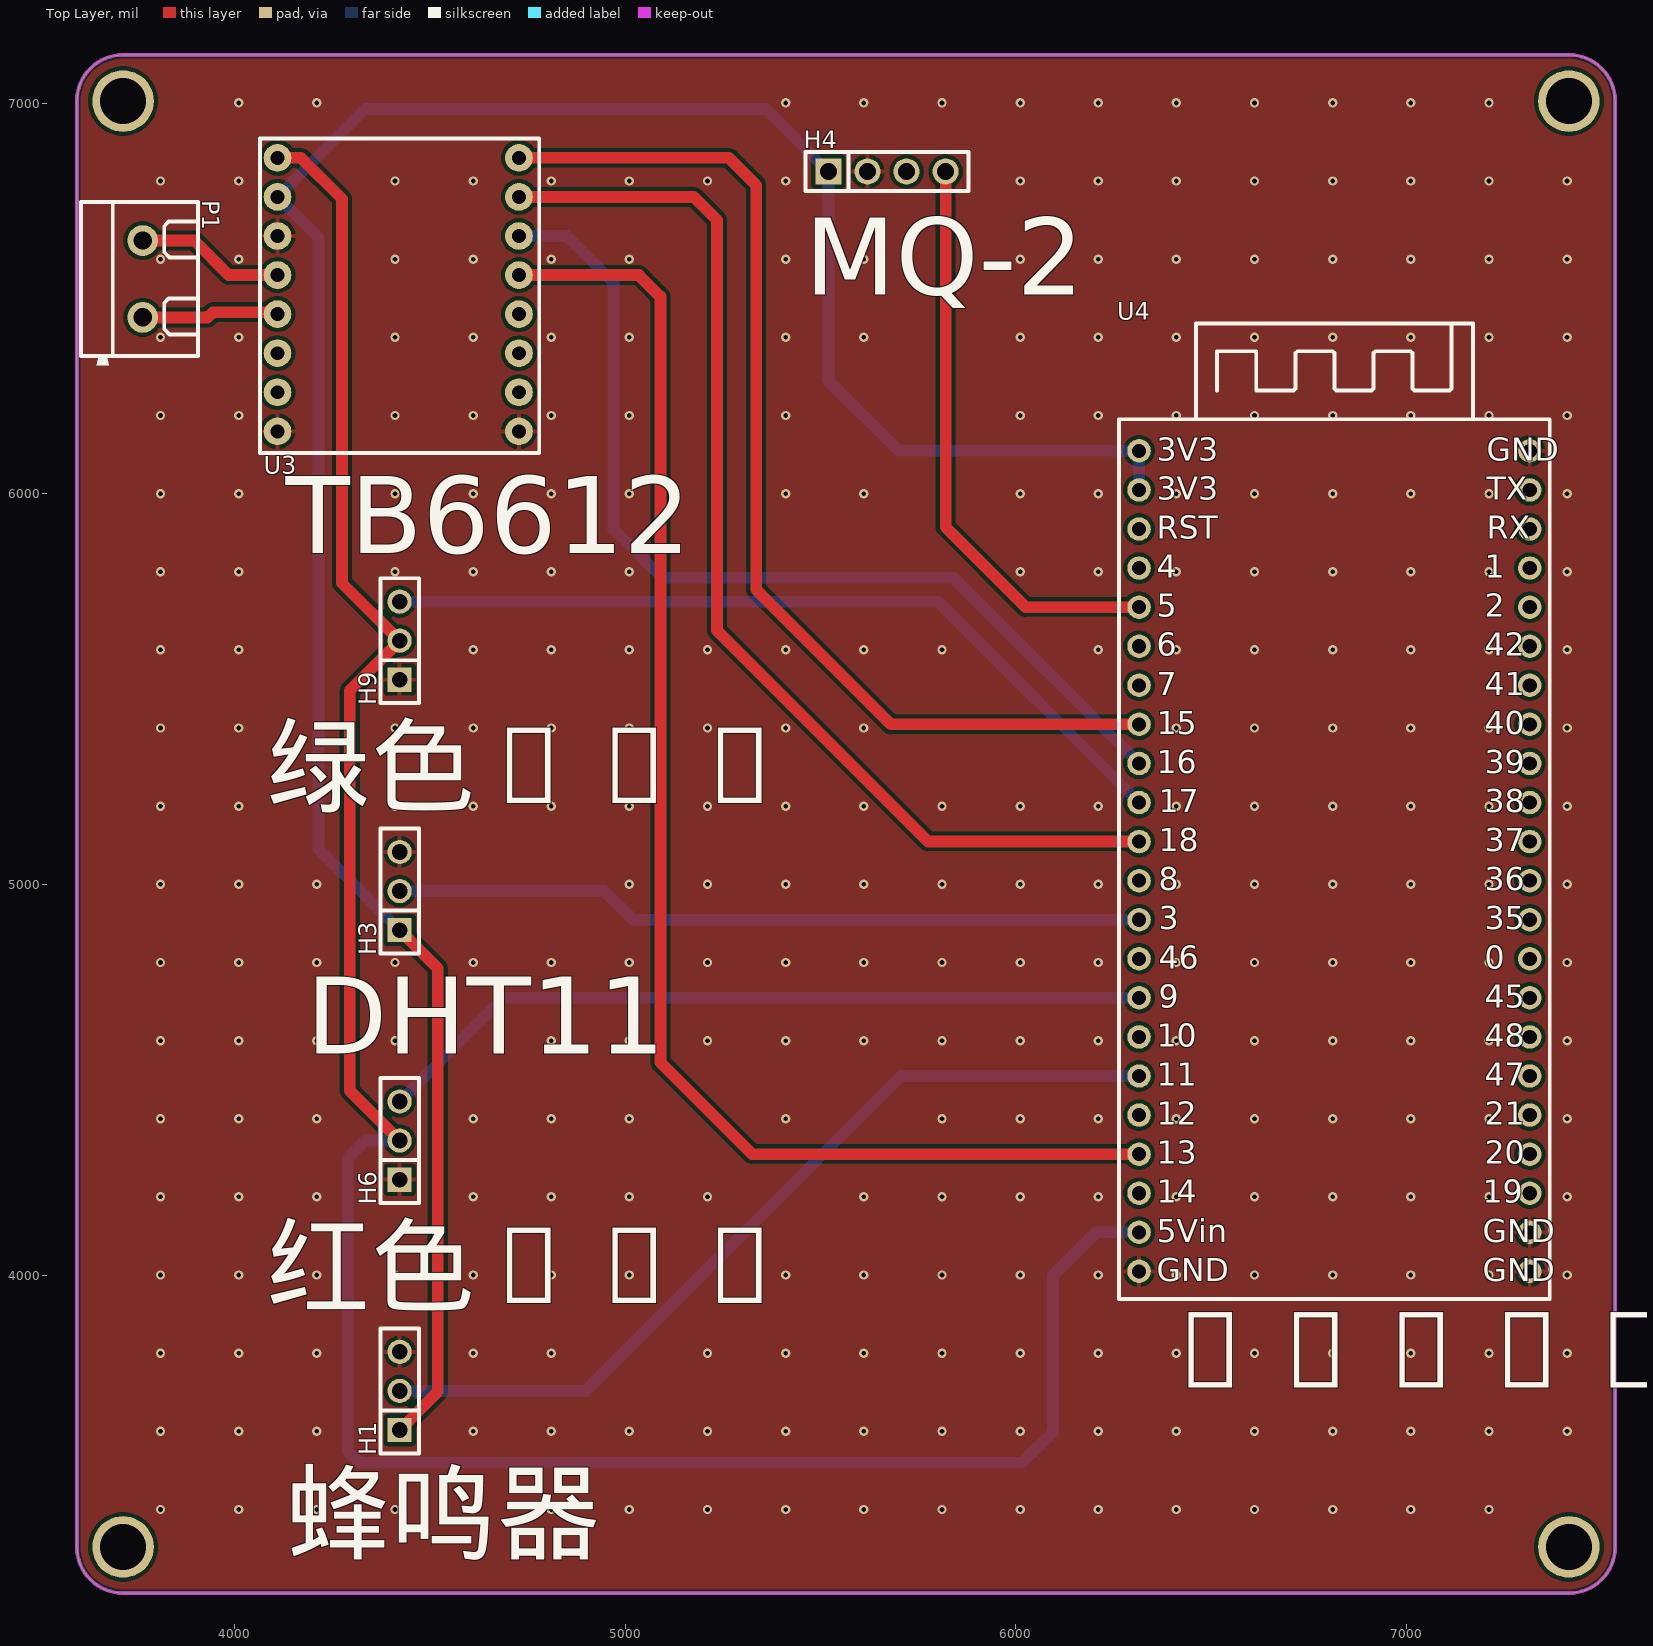
[diagram p0: Top Layer view]
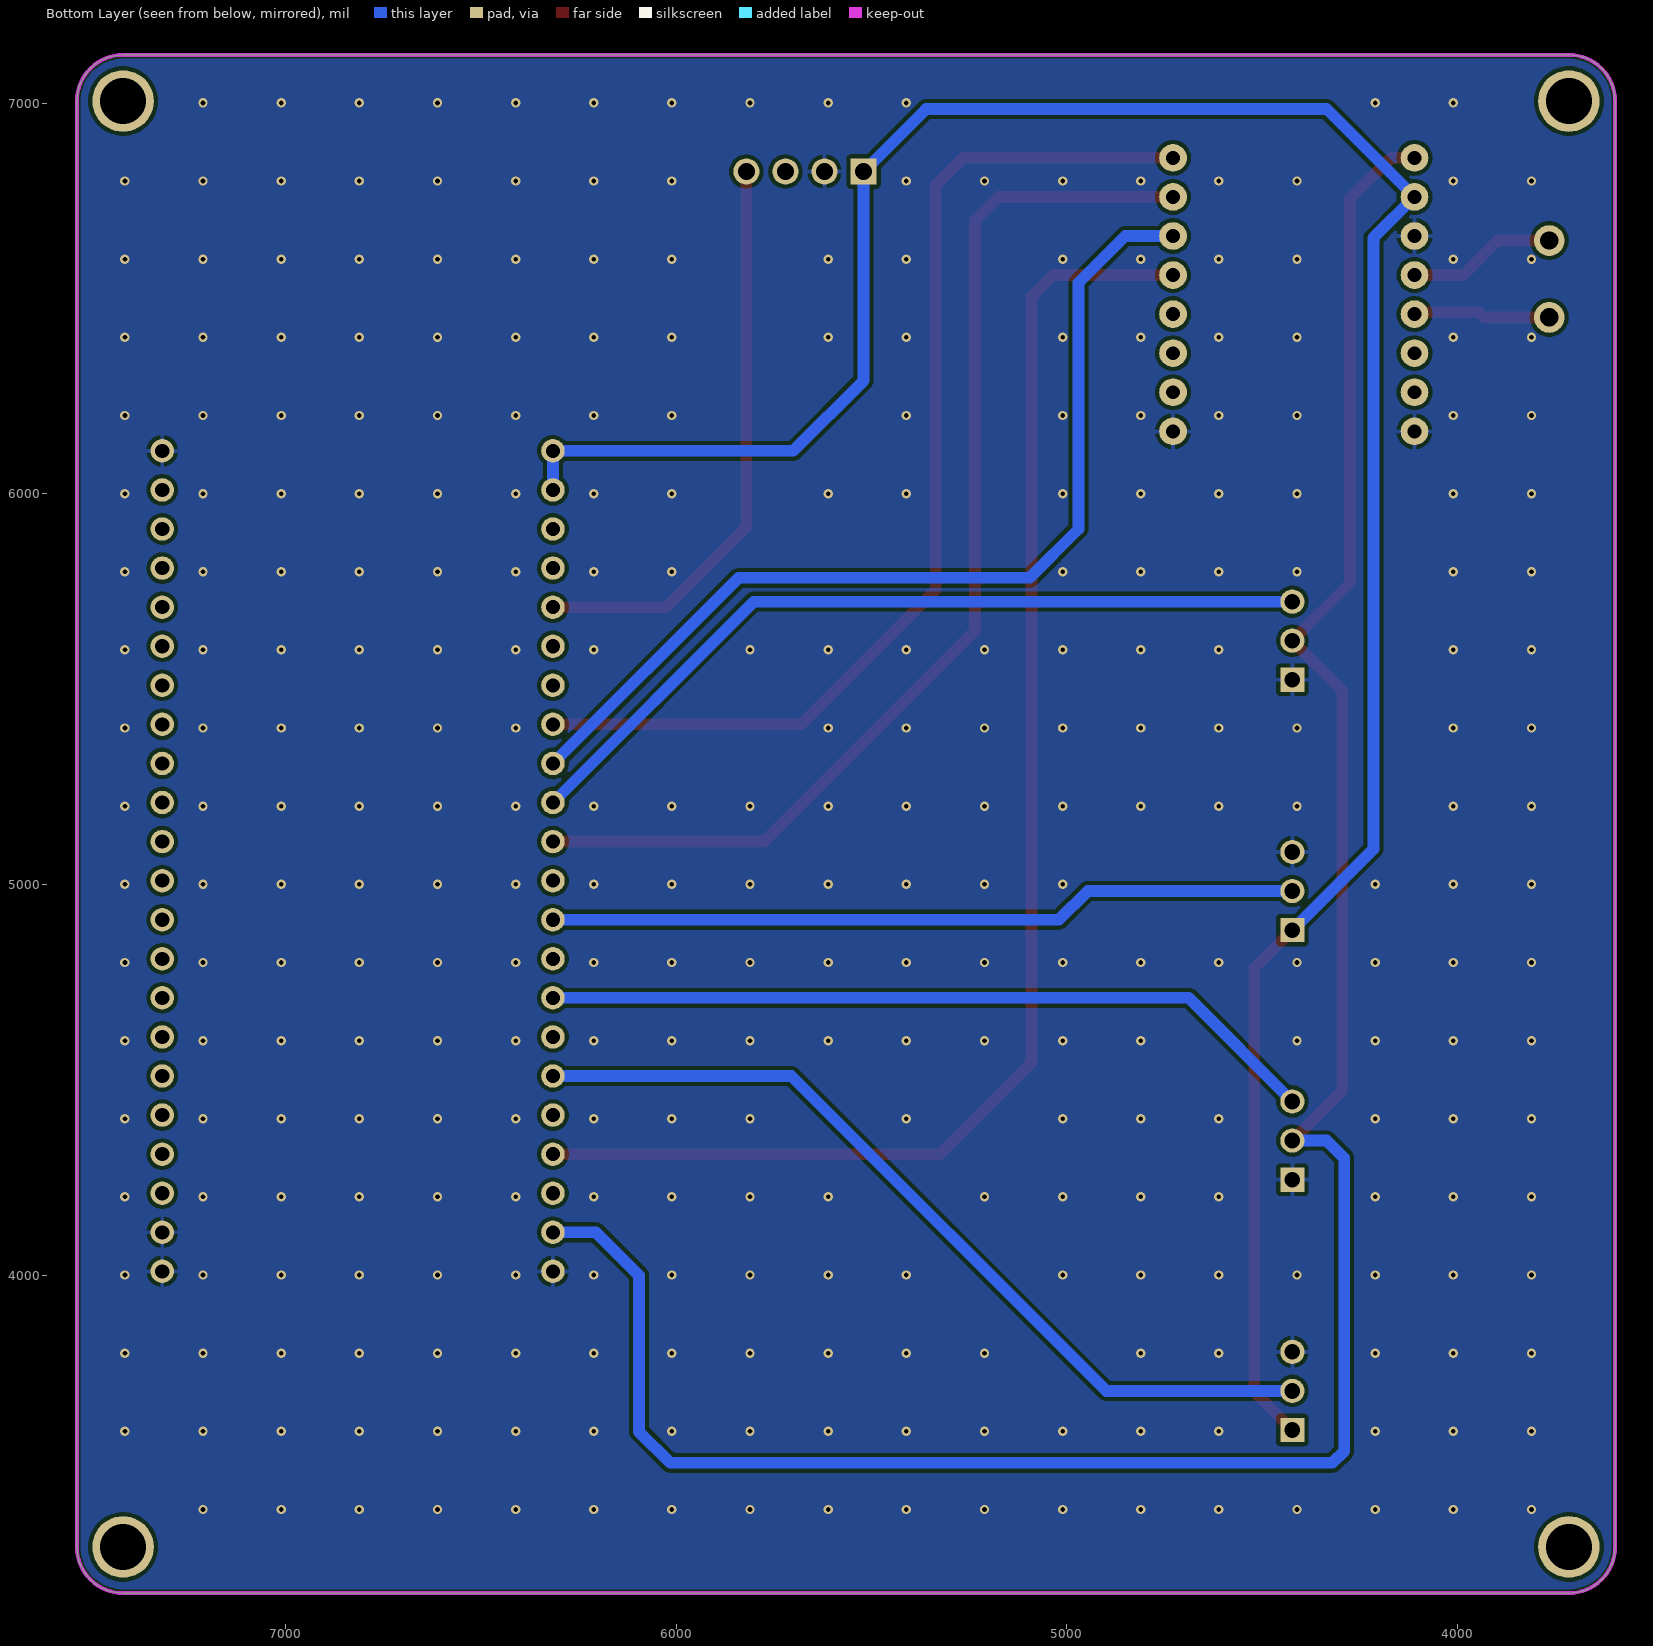
[diagram p1: Bottom Layer view, seen from below]
# Altium PCB MISC52005.pcbdoc
Units mil, origin at the board's own origin, x right, y up, seen from the top; angles counter-clockwise.
Board outline 3937.01 x 3937.01 mil, 2 copper layers (Top Layer, Bottom Layer), stack 62.206 mil thick; 8 components, 42 nets, 82 pads, 311 vias.

## Layer stack, top to bottom
Top Solder Mask Layer: solder mask 0.394, Dk 3.3
Top Layer: signal copper 1.379
Dielectric1: surface 59.449, FR4, Dk 4.5
Bottom Layer: signal copper 1.378
Bottom Solder Mask Layer: solder mask 0.394, Dk 3.3

## Board outline
3714.61,7123.5 ccw(c3714.61,7005.39) 3596.5,7005.39 3596.5,3304.61 ccw(c3714.61,3304.61) 3714.61,3186.5 7415.39,3186.5 ccw(c7415.39,3304.61) 7533.5,3304.61 7533.5,7005.39 ccw(c7415.39,7005.39) 7415.39,7123.5 3714.61,7123.5

## Design rules (kind name [scope] priority, off if disabled: settings)
BoardOutlineClearance copperThickness2oz_1 [All] p2 off: genericclearance=7.99 ignorepadtopadclearanceinfootprint=FALSE except(0: Arc-SplitContinuation Track-SplitContinuation SMDPad-SplitContinuation THPad-SplitContinuation Via-SplitContinuation Fill-SplitContinuation Region-SplitContinuation Poly-SplitContinuation Text-SplitContinuation Hole-SplitContinuation; 5.98: Arc-CutoutEdge Track-CutoutEdge SMDPad-CutoutEdge THPad-CutoutEdge Via-CutoutEdge Text-CutoutEdge; 6.9: Hole-OutlineEdge Hole-CutoutEdge; 10: Poly-OutlineEdge Poly-CutoutEdge; 11.81: Arc-OutlineEdge Track-OutlineEdge SMDPad-OutlineEdge THPad-OutlineEdge Via-OutlineEdge Fill-OutlineEdge Region-OutlineEdge Text-OutlineEdge Fill-CutoutEdge Region-CutoutEdge)
BoardOutlineClearance Plane_innerPlane_1 [All] p4 off: genericclearance=4.02 ignorepadtopadclearanceinfootprint=FALSE except(0: Arc-SplitContinuation Track-SplitContinuation SMDPad-SplitContinuation THPad-SplitContinuation Via-SplitContinuation Fill-SplitContinuation Region-SplitContinuation Poly-SplitContinuation Text-SplitContinuation Hole-SplitContinuation; 5.98: Arc-CutoutEdge Track-CutoutEdge SMDPad-CutoutEdge THPad-CutoutEdge Via-CutoutEdge Text-CutoutEdge; 6.9: Hole-OutlineEdge Hole-CutoutEdge; 10: Poly-OutlineEdge Poly-CutoutEdge; 11.81: Arc-OutlineEdge Track-OutlineEdge SMDPad-OutlineEdge THPad-OutlineEdge Via-OutlineEdge Fill-OutlineEdge Region-OutlineEdge Text-OutlineEdge Fill-CutoutEdge Region-CutoutEdge)
BoardOutlineClearance Copper_copperRegion_1 [All] p6 off: genericclearance=4.02 ignorepadtopadclearanceinfootprint=FALSE except(0: Arc-SplitContinuation Track-SplitContinuation SMDPad-SplitContinuation THPad-SplitContinuation Via-SplitContinuation Fill-SplitContinuation Region-SplitContinuation Poly-SplitContinuation Text-SplitContinuation Hole-SplitContinuation; 5.98: Arc-CutoutEdge Track-CutoutEdge SMDPad-CutoutEdge THPad-CutoutEdge Via-CutoutEdge Text-CutoutEdge; 6.9: Hole-OutlineEdge Hole-CutoutEdge; 10: Poly-OutlineEdge Poly-CutoutEdge; 11.81: Arc-OutlineEdge Track-OutlineEdge SMDPad-OutlineEdge THPad-OutlineEdge Via-OutlineEdge Fill-OutlineEdge Region-OutlineEdge Text-OutlineEdge Fill-CutoutEdge Region-CutoutEdge)
BoardOutlineClearance Copper_copperRegion_copperThickness1oz_1 [All] p8 off: genericclearance=4.02 ignorepadtopadclearanceinfootprint=FALSE except(0: Arc-SplitContinuation Track-SplitContinuation SMDPad-SplitContinuation THPad-SplitContinuation Via-SplitContinuation Fill-SplitContinuation Region-SplitContinuation Poly-SplitContinuation Text-SplitContinuation Hole-SplitContinuation; 5.98: Arc-CutoutEdge Track-CutoutEdge SMDPad-CutoutEdge THPad-CutoutEdge Via-CutoutEdge Text-CutoutEdge; 6.9: Hole-OutlineEdge Hole-CutoutEdge; 10: Poly-OutlineEdge Poly-CutoutEdge; 11.81: Arc-OutlineEdge Track-OutlineEdge SMDPad-OutlineEdge THPad-OutlineEdge Via-OutlineEdge Fill-OutlineEdge Region-OutlineEdge Text-OutlineEdge Fill-CutoutEdge Region-CutoutEdge)
BoardOutlineClearance Copper_copperRegion_Copper_copperRegion_1 [All] p10 off: genericclearance=4.02 ignorepadtopadclearanceinfootprint=FALSE except(0: Arc-SplitContinuation Track-SplitContinuation SMDPad-SplitContinuation THPad-SplitContinuation Via-SplitContinuation Fill-SplitContinuation Region-SplitContinuation Poly-SplitContinuation Text-SplitContinuation Hole-SplitContinuation; 5.98: Arc-CutoutEdge Track-CutoutEdge SMDPad-CutoutEdge THPad-CutoutEdge Via-CutoutEdge Text-CutoutEdge; 6.9: Hole-OutlineEdge Hole-CutoutEdge; 10: Poly-OutlineEdge Poly-CutoutEdge; 11.81: Arc-OutlineEdge Track-OutlineEdge SMDPad-OutlineEdge THPad-OutlineEdge Via-OutlineEdge Fill-OutlineEdge Region-OutlineEdge Text-OutlineEdge Fill-CutoutEdge Region-CutoutEdge)
BoardOutlineClearance copperThickness1oz_1 [All] p12: genericclearance=4.02 ignorepadtopadclearanceinfootprint=FALSE except(0: Arc-SplitContinuation Track-SplitContinuation SMDPad-SplitContinuation THPad-SplitContinuation Via-SplitContinuation Fill-SplitContinuation Region-SplitContinuation Poly-SplitContinuation Text-SplitContinuation Hole-SplitContinuation; 5.98: Arc-CutoutEdge Track-CutoutEdge SMDPad-CutoutEdge THPad-CutoutEdge Via-CutoutEdge Text-CutoutEdge; 6.9: Hole-OutlineEdge Hole-CutoutEdge; 10: Poly-OutlineEdge Poly-CutoutEdge; 11.81: Arc-OutlineEdge Track-OutlineEdge SMDPad-OutlineEdge THPad-OutlineEdge Via-OutlineEdge Fill-OutlineEdge Region-OutlineEdge Text-OutlineEdge Fill-CutoutEdge Region-CutoutEdge)
Clearance copperThickness2oz [All] p1 off: gap=7.99 ignorepadtopadclearanceinfootprint=FALSE except(5.98: SMDPad-Track SMDPad-SMDPad THPad-Track SMDPad-THPad THPad-THPad Track-Via SMDPad-Via THPad-Via Via-Via Fill-SMDPad Region-SMDPad Fill-THPad Region-THPad Fill-Via Region-Via Fill-Fill Fill-Region Region-Region Arc-Track Arc-SMDPad Arc-THPad Arc-Via Fill-Arc Region-Arc Arc-Arc Text-Track SMDPad-Text Text-THPad Text-Via Fill-Text Region-Text Arc-Text Text-Text; 6.9: Hole-Track Hole-SMDPad Hole-THPad Hole-Via Fill-Hole Region-Hole Hole-Arc Hole-Text; 10: Poly-Track Poly-SMDPad Poly-THPad Poly-Via Poly-Fill Poly-Region Poly-Poly Poly-Arc Poly-Text Poly-Hole; 11.81: Fill-Track Region-Track)
Clearance Plane_innerPlane [All] p3 off: gap=4.02 ignorepadtopadclearanceinfootprint=FALSE except(5.98: SMDPad-Track SMDPad-SMDPad THPad-Track SMDPad-THPad THPad-THPad Track-Via SMDPad-Via THPad-Via Via-Via Fill-SMDPad Region-SMDPad Fill-THPad Region-THPad Fill-Via Region-Via Fill-Fill Fill-Region Region-Region Arc-Track Arc-SMDPad Arc-THPad Arc-Via Fill-Arc Region-Arc Arc-Arc Text-Track SMDPad-Text Text-THPad Text-Via Fill-Text Region-Text Arc-Text Text-Text; 6.9: Hole-Track Hole-SMDPad Hole-THPad Hole-Via Fill-Hole Region-Hole Hole-Arc Hole-Text; 10: Poly-Track Poly-SMDPad Poly-THPad Poly-Via Poly-Fill Poly-Region Poly-Poly Poly-Arc Poly-Text Poly-Hole; 11.81: Fill-Track Region-Track)
Clearance Copper_copperRegion [All] p5 off: gap=4.02 ignorepadtopadclearanceinfootprint=FALSE except(5.98: SMDPad-Track SMDPad-SMDPad THPad-Track SMDPad-THPad THPad-THPad Track-Via SMDPad-Via THPad-Via Via-Via Fill-SMDPad Region-SMDPad Fill-THPad Region-THPad Fill-Via Region-Via Fill-Fill Fill-Region Region-Region Arc-Track Arc-SMDPad Arc-THPad Arc-Via Fill-Arc Region-Arc Arc-Arc Text-Track SMDPad-Text Text-THPad Text-Via Fill-Text Region-Text Arc-Text Text-Text; 6.9: Hole-Track Hole-SMDPad Hole-THPad Hole-Via Fill-Hole Region-Hole Hole-Arc Hole-Text; 10: Poly-Track Poly-SMDPad Poly-THPad Poly-Via Poly-Fill Poly-Region Poly-Poly Poly-Arc Poly-Text Poly-Hole; 11.81: Fill-Track Region-Track)
Clearance Copper_copperRegion_copperThickness1oz [All] p7 off: gap=4.02 ignorepadtopadclearanceinfootprint=FALSE except(5.98: SMDPad-Track SMDPad-SMDPad THPad-Track SMDPad-THPad THPad-THPad Track-Via SMDPad-Via THPad-Via Via-Via Fill-SMDPad Region-SMDPad Fill-THPad Region-THPad Fill-Via Region-Via Fill-Fill Fill-Region Region-Region Arc-Track Arc-SMDPad Arc-THPad Arc-Via Fill-Arc Region-Arc Arc-Arc Text-Track SMDPad-Text Text-THPad Text-Via Fill-Text Region-Text Arc-Text Text-Text; 6.9: Hole-Track Hole-SMDPad Hole-THPad Hole-Via Fill-Hole Region-Hole Hole-Arc Hole-Text; 10: Poly-Track Poly-SMDPad Poly-THPad Poly-Via Poly-Fill Poly-Region Poly-Poly Poly-Arc Poly-Text Poly-Hole; 11.81: Fill-Track Region-Track)
Clearance Copper_copperRegion_Copper_copperRegion [All] p9 off: gap=4.02 ignorepadtopadclearanceinfootprint=FALSE except(5.98: SMDPad-Track SMDPad-SMDPad THPad-Track SMDPad-THPad THPad-THPad Track-Via SMDPad-Via THPad-Via Via-Via Fill-SMDPad Region-SMDPad Fill-THPad Region-THPad Fill-Via Region-Via Fill-Fill Fill-Region Region-Region Arc-Track Arc-SMDPad Arc-THPad Arc-Via Fill-Arc Region-Arc Arc-Arc Text-Track SMDPad-Text Text-THPad Text-Via Fill-Text Region-Text Arc-Text Text-Text; 6.9: Hole-Track Hole-SMDPad Hole-THPad Hole-Via Fill-Hole Region-Hole Hole-Arc Hole-Text; 10: Poly-Track Poly-SMDPad Poly-THPad Poly-Via Poly-Fill Poly-Region Poly-Poly Poly-Arc Poly-Text Poly-Hole; 11.81: Fill-Track Region-Track)
Clearance copperThickness1oz [All] p11: gap=4.02 ignorepadtopadclearanceinfootprint=FALSE except(5.98: SMDPad-Track SMDPad-SMDPad THPad-Track SMDPad-THPad THPad-THPad Track-Via SMDPad-Via THPad-Via Via-Via Fill-SMDPad Region-SMDPad Fill-THPad Region-THPad Fill-Via Region-Via Fill-Fill Fill-Region Region-Region Arc-Track Arc-SMDPad Arc-THPad Arc-Via Fill-Arc Region-Arc Arc-Arc Text-Track SMDPad-Text Text-THPad Text-Via Fill-Text Region-Text Arc-Text Text-Text; 6.9: Hole-Track Hole-SMDPad Hole-THPad Hole-Via Fill-Hole Region-Hole Hole-Arc Hole-Text; 10: Poly-Track Poly-SMDPad Poly-THPad Poly-Via Poly-Fill Poly-Region Poly-Poly Poly-Arc Poly-Text Poly-Hole; 11.81: Fill-Track Region-Track)
DiffPairsRouting differentialPair [All] p1: maxlimit=6 minlimit=6 mostfreqgap=6 toplayer_minwidth=5 toplayer_prefwidth=10 toplayer_maxwidth=100 toplayer_mingap=6 toplayer_prefgap=6 toplayer_maxgap=6 bottomlayer_minwidth=5 bottomlayer_prefwidth=10 bottomlayer_maxwidth=100 bottomlayer_mingap=6 bottomlayer_prefgap=6 bottomlayer_maxgap=6 maxuncoupledlength=10
HoleToHoleClearance otherClearance [All] p1: gap=11.81 allowstackedmicrovias=TRUE
Length netLength [All] p1: minlimit=0 maxlimit=0
PasteMaskExpansion pasteMaskExpansion [All] p1: expansion=0
PlaneConnect innerPlane [All] p1: planeconnectstyle=Relief reliefexpansion=20 reliefentries=4 reliefconductorwidth=10 reliefairgap=10
PolygonConnect copperRegion_copperThickness1oz [All] p1 off: connectstyle=Relief reliefconductorwidth=10 reliefentries=4 polygonreliefangle="90 Angle" airgapwidth=10 via.connectstyle=Relief via.reliefconductorwidth=10 via.reliefentries=4 via.polygonreliefangle="90 Angle" via.airgapwidth=10
PolygonConnect copperRegion_Copper_copperRegion [All] p2 off: connectstyle=Relief reliefconductorwidth=10 reliefentries=4 polygonreliefangle="90 Angle" airgapwidth=10 via.connectstyle=Relief via.reliefconductorwidth=10 via.reliefentries=4 via.polygonreliefangle="90 Angle" via.airgapwidth=10
PolygonConnect copperRegion [All] p3: connectstyle=Relief reliefconductorwidth=10 reliefentries=4 polygonreliefangle="90 Angle" airgapwidth=10 via.connectstyle=Relief via.reliefconductorwidth=10 via.reliefentries=4 via.polygonreliefangle="90 Angle" via.airgapwidth=10
RoutingVias viaSize [All] p1: holewidth=12.01 width=24.02 viastyle="Through Hole" minholewidth=11.81 minwidth=19.68 maxholewidth=248.03 maxwidth=393.7
SolderMaskExpansion solderMaskExpansion [IsVia] p1: expansion=-1000 istentingtop=TRUE
SolderMaskExpansion solderMaskExpansion [All] p2: expansion=2 istentingtop=FALSE
Width copperThickness2oz_2 [All] p1 off: maxlimit=100 minlimit=8 preferedwidth=10
Width copperThickness1oz_2 [All] p2: maxlimit=100 minlimit=5 preferedwidth=10

## Components (designator, comment, footprint, x,y, rotation, side; value= is the part's Value field where it differs from the comment)
H1 "" HDR-TH_3P-P2.54-V-F 4422.5,3704.03 r90 top
H3 "" HDR-TH_3P-P2.54-V-F 4422.5,4983.39 r90 top
H4 "" HDR-TH_4P-P2.54-V-F 5670,6825 r0 top
H6 "" HDR-TH_3P-P2.54-V-F 4422.5,4344.75 r90 top
H9 "" HDR-TH_3P-P2.54-V-F 4422.5,5624.12 r90 top
P1 "KF301-2P接线端子" CONN-TH_XY301V-A-5.0-2P 3765,6550 r270 top
U3 "" tb6612 4110,6860 r0 top
U4 "NO" ESP32S3 6815,5065 r0 top

## Footprints (in the part's own frame and the unit in brackets; to place one, negate y for a bottom-side part, rotate by r counter-clockwise, add the part's x,y. Pads: shape width x height; smd on the part's side, far side on the other; paste and mask are expansions set on the pad)
CONN-TH_XY301V-A-5.0-2P [mm]
  round 2 hole 1.2: 1(-2.5,0) 2(2.5,0)
  silkscreen extent -5,-4 5.6,3.6
ESP32S3 [mil]
  round 60 hole 36: 1(-500,-1055) 2(-500,-955) 3(-500,-855) 4(-500,-755) 5(-500,-655) 6(-500,-555) 7(-500,-455) 8(-500,-355) 9(-500,-255) 10(-500,-155) 11(-500,-55) 12(-500,45) 13(-500,145) 14(-500,245) 15(-500,345) 16(-500,445) 17(-500,545) 18(-500,645) 19(-500,745) 20(-500,845) 21(-500,945) 22(-500,1045) 23(500,-1055) 24(500,-955) 25(500,-855) 26(500,-755) 27(500,-655) 28(500,-555) 29(500,-455) 30(500,-355) 31(500,-255) 32(500,-155) 33(500,-55) 34(500,45) 35(500,145) 36(500,245) 37(500,345) 38(500,445) 39(500,545) 40(500,645) 41(500,745) 42(500,845) 43(500,945) 44(500,1045)
  silkscreen extent -551,-1126 551,1371
HDR-TH_3P-P2.54-V-F [mil]
  rect 62x62 hole 40.16: 1(-100,0)
  round 62 hole 40.16: 2(0,0) 3(100,0)
  silkscreen extent -160,-49 160,49
HDR-TH_4P-P2.54-V-F [mm]
  rect 1.7x1.7 hole 1.1: 1(-3.81,0)
  round 1.7 hole 1.1: 2(-1.27,0) 3(1.27,0) 4(3.81,0)
  silkscreen extent -5.29,-1.27 5.29,1.27
tb6612 [mm]
  round 1.8 hole 0.9: 1(0,0) 2(0,-2.54) 3(0,-5.08) 4(0,-7.62) 5(0,-10.16) 6(0,-12.7) 7(0,-15.24) 8(0,-17.78) 9(15.697,-17.78) 10(15.697,-15.24) 11(15.697,-12.7) 12(15.697,-10.16) 13(15.697,-7.62) 14(15.697,-5.08) 15(15.697,-2.54) 16(15.697,0)
  silkscreen extent -1.14,-19.18 17.02,1.27

## Free pads (board coordinates)
  round 157.48 hole 118.11: 1(3714.61,7005.39) 1(3714.61,3304.61) 1(7415.39,7005.39) 1(7415.39,3304.61)

## Via types
v1: diameter 24.02, hole 12, Top Layer to Bottom Layer, 311 vias

## Nets (pads, with @x,y where several pads share a name; then routed paths per layer and width w, separated by ;. In a path a pad name is that pad's centre, name@x,y a point inside that pad or via, vN(x,y) a via of type N, cw(c..) or ccw(c..) an arc to the next point about the centre after c; other vN are vias at no path point)
0: U4.31
1: U4.41
2: U4.40
3: H3.2 U4.10 | length 1922.9
  Bottom Layer w30: H3.2 4946.61,4983.39 5020,4910 U4.10
4: U4.19
5: H4.4 U4.18 | length 1489.9
  Top Layer w30: H4.4 5820,5915 6025,5710 U4.18
6: U4.17
7: U4.16
8: U4.11
9: H6.3 U4.8 | length 2002.4
  Bottom Layer w30: H6.3 4687.75,4710 U4.8
10: U4.7
11: H1.2 U4.6 | length 2226.3
  Bottom Layer w30: H1.2 4899.03,3704.03 5705,4510 U4.6
12: U4.5
13: U3.13 U4.4 | length 3667.1
  Top Layer w30: U3.13 5035,6560 5090,6505 5090,4545 5325,4310 U4.4
14: U4.3
15: U3.16 U4.15 | length 2793.9
  Top Layer w30: U3.16 5265,6860 5335,6790 5335,5755 5680,5410 U4.15
16: U3.14 U4.14 | length 2515.2
  Bottom Layer w30: U3.14 4850,6660 4970,6540 4970,5910 5095,5785 5840,5785 U4.14
17: H9.3 U4.13 | length 2105.5
  Bottom Layer w30: H9.3 5800.88,5724.12 U4.13
18: U3.15 U4.12 | length 2885.5
  Top Layer w30: U3.15 5175,6760 5235,6700 5235,5650 5775,5110 U4.12
19: U4.25
20: U4.26
21: U4.27
35: U4.32
36: U4.33
37: U4.34
38: U4.35
39: U4.36
40: U4.37
41: U4.38
42: U4.39
45: U4.30
46: U4.9
47: U4.28
48: U4.29
$1N17300: P1.1 U3.4 | length 381.6
  Top Layer w30: P1.1 3896.57,6648.43 3985,6560 U3.4
$1N17301: P1.2 U3.5 | length 352.6
  Top Layer w30: P1.2 3931.57,6451.57 3945,6465 4105,6465 U3.5
+5V: H6.2 H9.2 U3.1 U4.2 | length 6202.6
  Top Layer w30: U3.1 4170,6860 4275,6755 4275,5771.62 H9.2 4295,5496.62 4295,4472.25 H6.2
  Bottom Layer w30: H6.2 4334.75,4344.75 4290,4300 4290,3550 4320,3520 6015,3520 6095,3600 6095,4000 6205,4110 U4.2
GND: H1.3 H3.3 H4.2 H6.1 H9.1 U3.3 U3.8 U3.9 U4.1 U4.23 U4.24 U4.44
  other v1: 3810.6,3400.6 4010.6,3400.6 4210.6,3400.6 4410.6,3400.6 4610.6,3400.6 4810.6,3400.6 5010.6,3400.6 5210.6,3400.6 5410.6,3400.6 5610.6,3400.6 5810.6,3400.6 6010.6,3400.6 6210.6,3400.6 6410.6,3400.6 6610.6,3400.6 6810.6,3400.6 7010.6,3400.6 7210.6,3400.6 3810.6,3600.6 4010.6,3600.6 4210.6,3600.6 4610.6,3600.6 4810.6,3600.6 5010.6,3600.6 5210.6,3600.6 5410.6,3600.6 5610.6,3600.6 5810.6,3600.6 6010.6,3600.6 6210.6,3600.6 6410.6,3600.6 6610.6,3600.6 6810.6,3600.6 7010.6,3600.6 7210.6,3600.6 7410.6,3600.6 3810.6,3800.6 4010.6,3800.6 4210.6,3800.6 4610.6,3800.6 4810.6,3800.6 5210.6,3800.6 5410.6,3800.6 5610.6,3800.6 5810.6,3800.6 6010.6,3800.6 6210.6,3800.6 6410.6,3800.6 6610.6,3800.6 6810.6,3800.6 7010.6,3800.6 7210.6,3800.6 7410.6,3800.6 3810.6,4000.6 4010.6,4000.6 4210.6,4000.6 4410.6,4000.6 4610.6,4000.6 4810.6,4000.6 5010.6,4000.6 5410.6,4000.6 5610.6,4000.6 5810.6,4000.6 6010.6,4000.6 6210.6,4000.6 6410.6,4000.6 6610.6,4000.6 6810.6,4000.6 7010.6,4000.6 7210.6,4000.6 7410.6,4000.6 3810.6,4200.6 4010.6,4200.6 4210.6,4200.6 4610.6,4200.6 4810.6,4200.6 5010.6,4200.6 5210.6,4200.6 5610.6,4200.6 5810.6,4200.6 6010.6,4200.6 6210.6,4200.6 6410.6,4200.6 6610.6,4200.6 6810.6,4200.6 7010.6,4200.6 7210.6,4200.6 7410.6,4200.6 3810.6,4400.6 4010.6,4400.6 4210.6,4400.6 4610.6,4400.6 4810.6,4400.6 5010.6,4400.6 5410.6,4400.6 5810.6,4400.6 6010.6,4400.6 6210.6,4400.6 6410.6,4400.6 6610.6,4400.6 6810.6,4400.6 7010.6,4400.6 7210.6,4400.6 7410.6,4400.6 3810.6,4600.6 4010.6,4600.6 4210.6,4600.6 4410.6,4600.6 4810.6,4600.6 5010.6,4600.6 5210.6,4600.6 5410.6,4600.6 5610.6,4600.6 5810.6,4600.6 6010.6,4600.6 6210.6,4600.6 6410.6,4600.6 6610.6,4600.6 6810.6,4600.6 7010.6,4600.6 7210.6,4600.6 7410.6,4600.6 3810.6,4800.6 4010.6,4800.6 4210.6,4800.6 4410.6,4800.6 4610.6,4800.6 4810.6,4800.6 5010.6,4800.6 5210.6,4800.6 5410.6,4800.6 5610.6,4800.6 5810.6,4800.6 6010.6,4800.6 6210.6,4800.6 6410.6,4800.6 6610.6,4800.6 6810.6,4800.6 7010.6,4800.6 7210.6,4800.6 7410.6,4800.6 3810.6,5000.6 4010.6,5000.6 4210.6,5000.6 5010.6,5000.6 5210.6,5000.6 5410.6,5000.6 5610.6,5000.6 5810.6,5000.6 6010.6,5000.6 6210.6,5000.6 6410.6,5000.6 6610.6,5000.6 6810.6,5000.6 7010.6,5000.6 7210.6,5000.6 7410.6,5000.6 3810.6,5200.6 4010.6,5200.6 4410.6,5200.6 4610.6,5200.6 4810.6,5200.6 5010.6,5200.6 5210.6,5200.6 5410.6,5200.6 5610.6,5200.6 5810.6,5200.6 6010.6,5200.6 6210.6,5200.6 6410.6,5200.6 6610.6,5200.6 6810.6,5200.6 7010.6,5200.6 7210.6,5200.6 7410.6,5200.6 3810.6,5400.6 4010.6,5400.6 4410.6,5400.6 4610.6,5400.6 4810.6,5400.6 5010.6,5400.6 5210.6,5400.6 5410.6,5400.6 5610.6,5400.6 6410.6,5400.6 6610.6,5400.6 6810.6,5400.6 7010.6,5400.6 7210.6,5400.6 7410.6,5400.6 3810.6,5600.6 4010.6,5600.6 4610.6,5600.6 4810.6,5600.6 5010.6,5600.6 5210.6,5600.6 5410.6,5600.6 5610.6,5600.6 5810.6,5600.6 6210.6,5600.6 6410.6,5600.6 6610.6,5600.6 6810.6,5600.6 7010.6,5600.6 7210.6,5600.6 7410.6,5600.6 3810.6,5800.6 4010.6,5800.6 4410.6,5800.6 4610.6,5800.6 4810.6,5800.6 5010.6,5800.6 6010.6,5800.6 6210.6,5800.6 6410.6,5800.6 6610.6,5800.6 6810.6,5800.6 7010.6,5800.6 7210.6,5800.6 7410.6,5800.6 3810.6,6000.6 4010.6,6000.6 4410.6,6000.6 4610.6,6000.6 4810.6,6000.6 5010.6,6000.6 5410.6,6000.6 5610.6,6000.6 6010.6,6000.6 6210.6,6000.6 6410.6,6000.6 6610.6,6000.6 6810.6,6000.6 7010.6,6000.6 7210.6,6000.6 7410.6,6000.6 3810.6,6200.6 4010.6,6200.6 4410.6,6200.6 4610.6,6200.6 4810.6,6200.6 5010.6,6200.6 5410.6,6200.6 6010.6,6200.6 6210.6,6200.6 6410.6,6200.6 6610.6,6200.6 6810.6,6200.6 7010.6,6200.6 7210.6,6200.6 7410.6,6200.6 3810.6,6400.6 4010.6,6400.6 4410.6,6400.6 4610.6,6400.6 4810.6,6400.6 5010.6,6400.6 5410.6,6400.6 5610.6,6400.6 6010.6,6400.6 6210.6,6400.6 6410.6,6400.6 6610.6,6400.6 6810.6,6400.6 7010.6,6400.6 7210.6,6400.6 7410.6,6400.6 3810.6,6600.6 4010.6,6600.6 4410.6,6600.6 4610.6,6600.6 4810.6,6600.6 5010.6,6600.6 5410.6,6600.6 5610.6,6600.6 6010.6,6600.6 6210.6,6600.6 6410.6,6600.6 6610.6,6600.6 6810.6,6600.6 7010.6,6600.6 7210.6,6600.6 7410.6,6600.6 3810.6,6800.6 4010.6,6800.6 4410.6,6800.6 4610.6,6800.6 4810.6,6800.6 5010.6,6800.6 5210.6,6800.6 5410.6,6800.6 6010.6,6800.6 6210.6,6800.6 6410.6,6800.6 6610.6,6800.6 6810.6,6800.6 7010.6,6800.6 7210.6,6800.6 7410.6,6800.6 4010.6,7000.6 4210.6,7000.6 5410.6,7000.6 5610.6,7000.6 5810.6,7000.6 6010.6,7000.6 6210.6,7000.6 6410.6,7000.6 6610.6,7000.6 6810.6,7000.6 7010.6,7000.6 7210.6,7000.6
RST: U4.20
RX: U4.42
TX: U4.43
VCC: H1.1 H3.1 H4.1 U3.2 U4.21 U4.22 | length 6440.2
  Top Layer w30: H1.1 4520,3701.53 4520,4785.89 H3.1
  Bottom Layer w30: H3.1 4215,5090.89 4215,6655 U3.2 4335,6985 5360,6985 H4.1 5520,6290 5700,6110 U4.22 U4.21
pads on no net: H4.3 U3.6 U3.7 U3.10 U3.11 U3.12

## Polygon pours and split planes (outlines as drawn)
GND on Bottom Layer (solid, remove dead copper, pour order 2): 3525,7245 3525,3080 7700,3080 7700,7245
GND on Top Layer (solid, remove dead copper, pour order 2): 3000,7415 3000,3000 7930,3000 7930,7415

## Keep-outs
Board Outline Layer:
  the board outline again, w10

## Silkscreen, mask and mechanical layers (free items; w line width, h text height)
Top Silkscreen Layer:
  text "MQ-2" at 5460,6510 h196.85
  text "TB6612" at 4130.8,5847.84 h196.85
  text "绿色LED" at 4078.61,5208.31 h196.85
  text "DHT11" at 4183.89,4566.69 h196.85
  text "红色LED" at 4078.91,3928.95 h196.85
  text "ESP32-S3开发板" at 6362.87,3711.57 h196.85
  text "蜂鸣器" at 4129.31,3296.57 h196.85